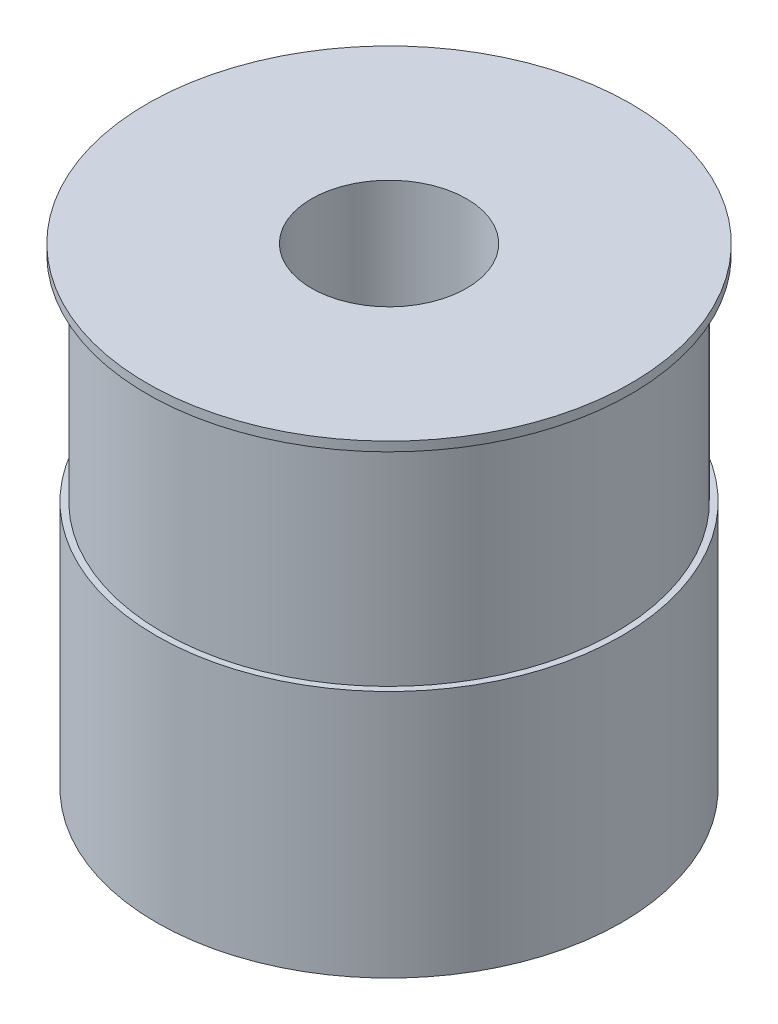
from build123d import *


with BuildPart() as part:
    # 草图1 → 旋转1 (revolve)
    with BuildSketch(Plane.XY, mode=Mode.PRIVATE) as revolve_1_sk:
        Polygon((-37.5, 0), (-37.5, 40), (-36.5, 40), (-36.5, 74.5), (-39, 74.5), (-39, 76), (-17.5, 76), (-12.5, 76), (-12.5, 51), (-17.5, 51), (-17.5, 36), (-30, 36), (-30, 33), (-32.5, 33), (-32.5, 0), align=None)
    revolve(revolve_1_sk.sketch.rotate(Axis((0, 0, 0), (0, 1, 0)), 270), axis=Axis((0, 0, 0), (0, 1, 0)))


solid = part.part
